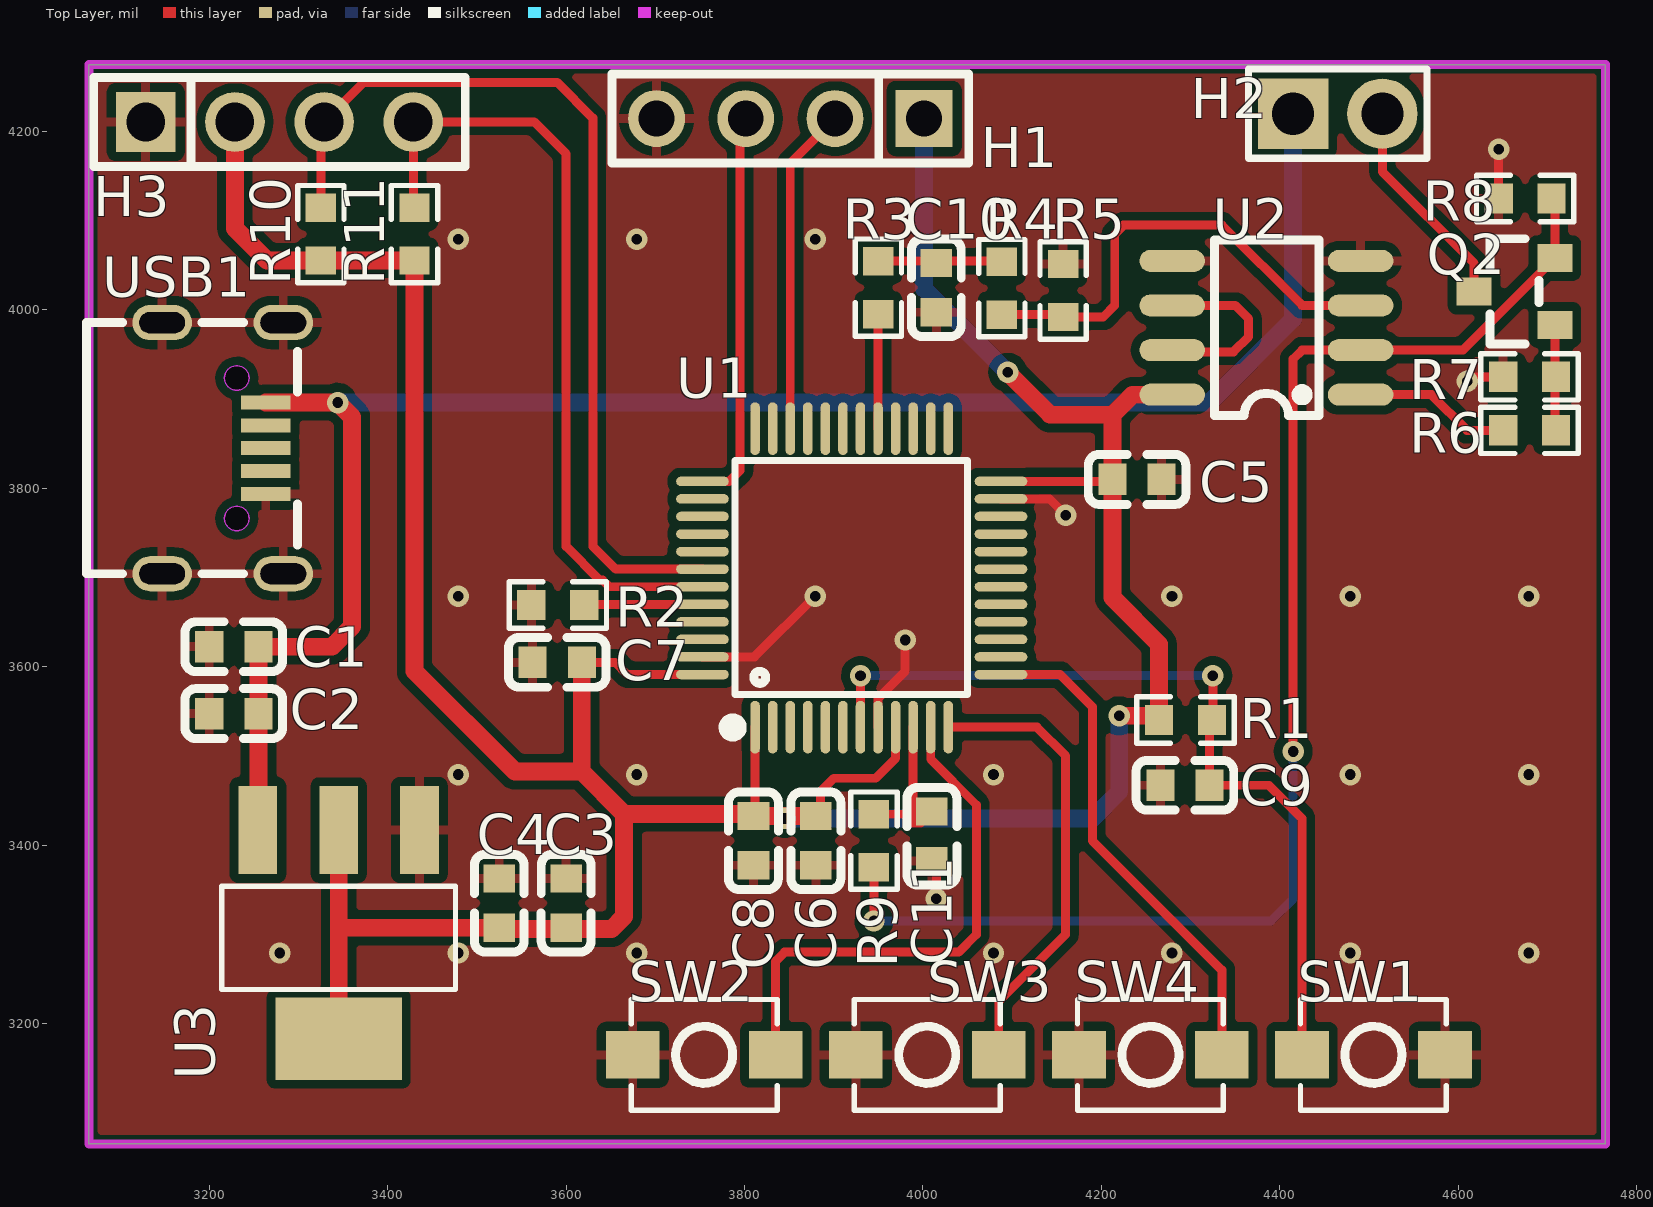
[diagram p0: Top Layer view]
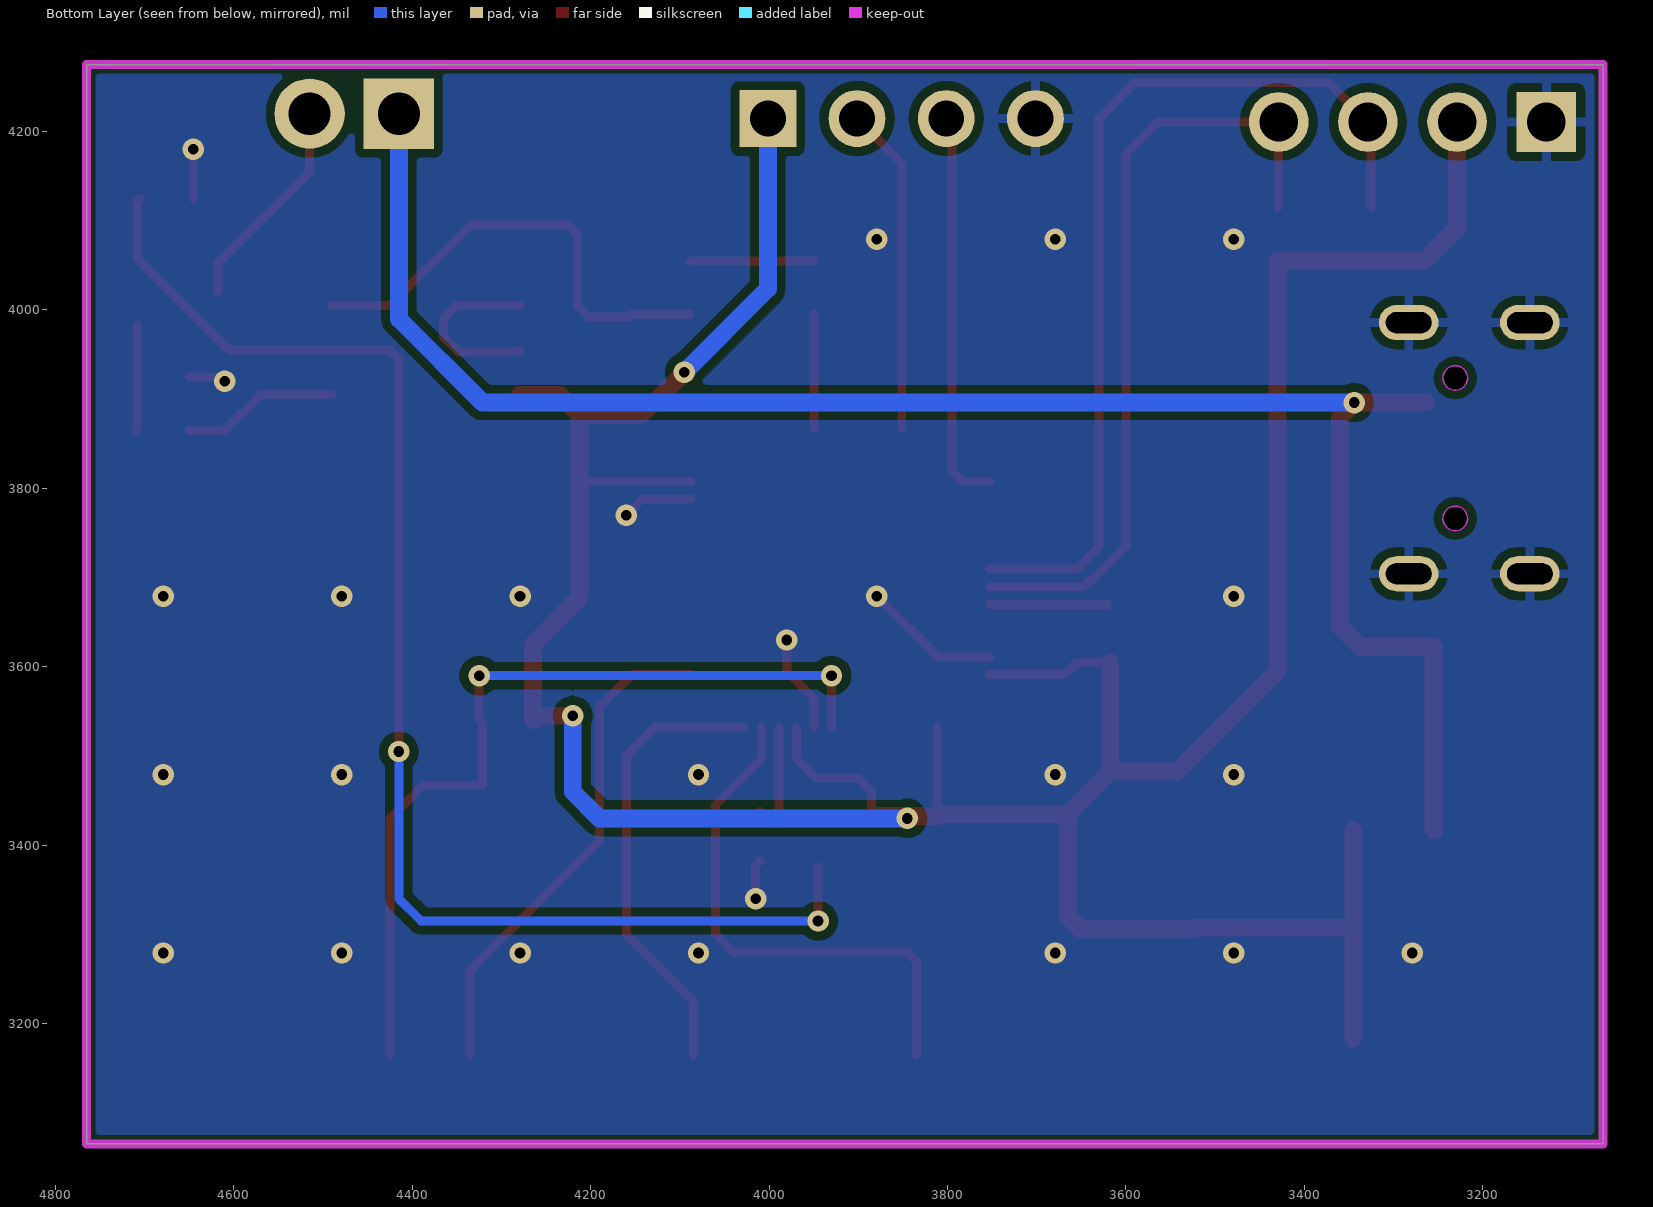
[diagram p1: Bottom Layer view, seen from below]
# Altium PCB MISC52008.pcbdoc
Units mil, origin at the board's own origin, x right, y up, seen from the top; angles counter-clockwise.
Board outline 1700 x 1210 mil, 2 copper layers (Top Layer, Bottom Layer), stack 62.206 mil thick; 34 components, 21 nets, 134 pads, 33 vias.

## Layer stack, top to bottom
Top Solder Mask Layer: solder mask 0.394, Dk 3.3
Top Layer: signal copper 1.379
Dielectric1: surface 59.449, FR4, Dk 4.5
Bottom Layer: signal copper 1.378
Bottom Solder Mask Layer: solder mask 0.394, Dk 3.3

## Board outline
3065,4275 3065,3065 4765,3065 4765,4275

## Design rules (kind name [scope] priority, off if disabled: settings)
BoardOutlineClearance copperThickness2oz_1 [All] p2 off: genericclearance=7.99 ignorepadtopadclearanceinfootprint=FALSE except(0: Arc-SplitContinuation Track-SplitContinuation SMDPad-SplitContinuation THPad-SplitContinuation Via-SplitContinuation Fill-SplitContinuation Region-SplitContinuation Poly-SplitContinuation Text-SplitContinuation Hole-SplitContinuation; 5.98: Arc-CutoutEdge SMDPad-CutoutEdge THPad-CutoutEdge Via-CutoutEdge Fill-CutoutEdge Region-CutoutEdge Text-CutoutEdge; 6.93: Hole-OutlineEdge Hole-CutoutEdge; 10: Poly-OutlineEdge Poly-CutoutEdge; 11.81: Arc-OutlineEdge Track-OutlineEdge SMDPad-OutlineEdge THPad-OutlineEdge Via-OutlineEdge Fill-OutlineEdge Region-OutlineEdge Text-OutlineEdge Track-CutoutEdge)
BoardOutlineClearance copperThickness1oz_1 [All] p4: genericclearance=4.02 ignorepadtopadclearanceinfootprint=FALSE except(0: Arc-SplitContinuation Track-SplitContinuation SMDPad-SplitContinuation THPad-SplitContinuation Via-SplitContinuation Fill-SplitContinuation Region-SplitContinuation Poly-SplitContinuation Text-SplitContinuation Hole-SplitContinuation; 6: SMDPad-CutoutEdge THPad-CutoutEdge Via-CutoutEdge Fill-CutoutEdge Region-CutoutEdge Text-CutoutEdge; 6.93: Hole-OutlineEdge Hole-CutoutEdge; 10: Poly-OutlineEdge Poly-CutoutEdge; 11.8: Arc-OutlineEdge Track-OutlineEdge SMDPad-OutlineEdge THPad-OutlineEdge Via-OutlineEdge Fill-OutlineEdge Region-OutlineEdge Text-OutlineEdge; 11.81: Arc-CutoutEdge Track-CutoutEdge)
Clearance copperThickness2oz [All] p1 off: gap=7.99 ignorepadtopadclearanceinfootprint=FALSE except(5.98: SMDPad-Track SMDPad-SMDPad THPad-Track SMDPad-THPad THPad-THPad Track-Via SMDPad-Via THPad-Via Via-Via Fill-Track Region-Track Fill-SMDPad Region-SMDPad Fill-THPad Region-THPad Fill-Via Region-Via Fill-Fill Fill-Region Region-Region Arc-Track Arc-SMDPad Arc-THPad Arc-Via Fill-Arc Region-Arc Arc-Arc Text-Track SMDPad-Text Text-THPad Text-Via Fill-Text Region-Text Arc-Text Text-Text; 6.93: Hole-Track Hole-SMDPad Hole-THPad Hole-Via Fill-Hole Region-Hole Hole-Arc Hole-Text; 10: Poly-Track Poly-SMDPad Poly-THPad Poly-Via Poly-Fill Poly-Region Poly-Poly Poly-Arc Poly-Text Poly-Hole)
Clearance copperThickness1oz [All] p3: gap=4.02 ignorepadtopadclearanceinfootprint=FALSE except(5.98: SMDPad-Track SMDPad-SMDPad THPad-Track SMDPad-THPad THPad-THPad Track-Via SMDPad-Via THPad-Via Via-Via Fill-Track Region-Track Fill-SMDPad Region-SMDPad Fill-THPad Region-THPad Fill-Via Region-Via Fill-Fill Fill-Region Region-Region; 6: Arc-Track Arc-SMDPad Arc-THPad Arc-Via Fill-Arc Region-Arc Arc-Arc Text-Track SMDPad-Text Text-THPad Text-Via Fill-Text Region-Text Arc-Text Text-Text; 6.93: Hole-Track Hole-SMDPad Hole-THPad Hole-Via Fill-Hole Region-Hole Hole-Arc Hole-Text; 10: Poly-Track Poly-SMDPad Poly-THPad Poly-Via Poly-Fill Poly-Region Poly-Poly Poly-Arc Poly-Text Poly-Hole)
DiffPairsRouting differentialPair [All] p1: maxlimit=6 minlimit=6 mostfreqgap=6 toplayer_minwidth=5 toplayer_prefwidth=10 toplayer_maxwidth=100 toplayer_mingap=6 toplayer_prefgap=6 toplayer_maxgap=6 bottomlayer_minwidth=5 bottomlayer_prefwidth=10 bottomlayer_maxwidth=100 bottomlayer_mingap=6 bottomlayer_prefgap=6 bottomlayer_maxgap=6 maxuncoupledlength=10
HoleToHoleClearance otherClearance [All] p1: gap=11.81 allowstackedmicrovias=TRUE
Length netLength [All] p1: minlimit=0 maxlimit=0
MatchedLengths netLengthTolerance [All] p1: tolerance=1000
PasteMaskExpansion pasteMaskExpansion [All] p1: expansion=0
PlaneConnect innerPlane [All] p1: planeconnectstyle=Relief reliefexpansion=20 reliefentries=4 reliefconductorwidth=10 reliefairgap=10
PolygonConnect copperRegion [(InNet('GND'))] p1: connectstyle=Relief reliefconductorwidth=10 reliefentries=4 polygonreliefangle="90 Angle" airgapwidth=10 via.connectstyle=Relief via.reliefconductorwidth=10 via.reliefentries=4 via.polygonreliefangle="90 Angle" via.airgapwidth=10
RoutingVias viaSize [All] p1: holewidth=12.01 width=24.02 viastyle="Through Hole" minholewidth=11.81 minwidth=19.68 maxholewidth=248.03 maxwidth=393.7
SolderMaskExpansion solderMaskExpansion [IsVia] p1: expansion=-1000 istentingtop=TRUE
SolderMaskExpansion solderMaskExpansion [All] p2: expansion=2 istentingtop=FALSE
Width copperThickness2oz_2 [All] p1 off: maxlimit=100 minlimit=8 preferedwidth=10
Width copperThickness1oz_2 [All] p2: maxlimit=100 minlimit=5 preferedwidth=10

## Components (designator, comment, footprint, x,y, rotation, side; value= is the part's Value field where it differs from the comment)
C1 "10uf" C0603 3227.5,3622.5 r0 top
C2 "0.1uf" C0603 3227.5,3547.5 r0 top
C3 "10uf" C0603 3600,3335 r270 top
C4 "0.1uf" C0603 3525,3335 r270 top
C5 "0.1uf" C0603 4240,3810 r180 top
C6 "0.1uf" C0603 3880,3405 r90 top
C7 "0.1uf" C0603 3590,3605 r0 top
C8 "0.1uf" C0603 3810,3405 r90 top
C9 "0.1uf" C0603 4293.67,3467.16 r0 top
C10 "1uf" C0603 4015,4025 r270 top
C11 "100nF" C0603 4010,3410 r90 top
H1 "HX PH254-01-04-Z-L11.5 straight pin header" HDR-TH_4P-HX-PH254-01-04-Z-L11.5 3851.34,4214.55 r180 top
H2 "HX PH254-01-02-Z-L11.5 male header connector" HDR-TH_2P-P2.54-V-M 4465,4220 r0 top
H3 "2.54-1*4P female" HDR-TH_4P-P2.54-V-F 3278.67,4210.72 r0 top
Q2 "AO3400" SOT-23_L2.9-W1.3-P1.90-LS2.4-BR 4663.04,4020.72 r0 top
R1 "10K" R0603 4294.35,3540.26 r180 top
R2 "100K" R0603 3590.66,3669.2 r180 top
R3 "10K" R0603 3950,4025 r90 top
R4 "3.3k" R0603 4088.39,4024.39 r270 top
R5 "5.1k" R0603 4157.2,4021.75 r90 top
R6 "100" R0603 4680,3865 r0 top
R7 "100K" R0603 4680,3925 r0 top
R8 "10K" R0603 4675,4125 r0 top
R9 "10K" R0603 3945,3405 r90 top
R10 "4.7K" R0603 3325,4085 r90 top
R11 "4.7K" R0603 3430,4085 r90 top
SW1 "" Key_SMD_3x4x2 4505,3165 r0 top
SW2 "" Key_SMD_3x4x2 3754.79,3165 r180 top
SW3 "" Key_SMD_3x4x2 4004.86,3165 r180 top
SW4 "" Key_SMD_3x4x2 4254.93,3165 r180 top
U1 "AT32F421C8T7" LQFP-48_L7.0-W7.0-P0.50-LS9.0-BL 3920.11,3699.55 r0 top
U2 "LMV358" SOP-8_L4.9-W3.9-P1.27-LS6.0-BL 4385,3980 r90 top
U3 "AMS1117-3.3(XBLW)" SOT-223-3_L6.5-W3.4-P2.30-LS7.0-BR-1 3345,3300 r90 top
USB1 "" USB_Micro 3215,3845 r270 top

## Footprints (in the part's own frame and the unit in brackets; to place one, negate y for a bottom-side part, rotate by r counter-clockwise, add the part's x,y. Pads: shape width x height; smd on the part's side, far side on the other; paste and mask are expansions set on the pad)
C0603 [mm]
  rect 0.8x0.9 smd: 1(-0.7,0) 2(0.7,0)
  silkscreen extent -1.39,-0.71 1.39,0.71
HDR-TH_2P-P2.54-V-M [mm]
  rect 2x2 hole 1.2: 1(-1.27,0)
  round 2 hole 1.2: 2(1.27,0)
  silkscreen extent -2.54,-1.27 2.54,1.27
HDR-TH_4P-HX-PH254-01-04-Z-L11.5 [mm]
  rect 1.62x1.62 hole 1.02: 1(-3.81,0)
  round 1.62 hole 1.02: 2(-1.27,0) 3(1.27,0) 4(3.81,0)
  silkscreen extent -5.08,-1.27 5.08,1.27
HDR-TH_4P-P2.54-V-F [mm]
  rect 1.7x1.7 hole 1.1: 1(-3.81,0)
  round 1.7 hole 1.1: 2(-1.27,0) 3(1.27,0) 4(3.81,0)
  silkscreen extent -5.29,-1.27 5.29,1.27
Key_SMD_3x4x2 [mm]
  rect 1.53x1.36 smd paste+0 mask+0.051: 1(-2.035,0) 2(2.035,0)
  silkscreen extent -2.08,-1.58 2.08,1.58
LQFP-48_L7.0-W7.0-P0.50-LS9.0-BL [mm]
  oval 0.27x1.5 smd paste+0 mask+0.05: 1(-2.75,-4.25) 2(-2.25,-4.25) 3(-1.75,-4.25) 4(-1.25,-4.25) 5(-0.75,-4.25) 6(-0.25,-4.25) 7(0.25,-4.25) 8(0.75,-4.25) 9(1.25,-4.25) 10(1.75,-4.25) 11(2.25,-4.25) 12(2.75,-4.25) 25(2.75,4.25) 26(2.25,4.25) 27(1.75,4.25) 28(1.25,4.25) 29(0.75,4.25) 30(0.25,4.25) 31(-0.25,4.25) 32(-0.75,4.25) 33(-1.25,4.25) 34(-1.75,4.25) 35(-2.25,4.25) 36(-2.75,4.25)
  oval 1.5x0.27 smd paste+0 mask+0.05: 13(4.25,-2.75) 14(4.25,-2.25) 15(4.25,-1.75) 16(4.25,-1.25) 17(4.25,-0.75) 18(4.25,-0.25) 19(4.25,0.25) 20(4.25,0.75) 21(4.25,1.25) 22(4.25,1.75) 23(4.25,2.25) 24(4.25,2.75) 37(-4.25,2.75) 38(-4.25,2.25) 39(-4.25,1.75) 40(-4.25,1.25) 41(-4.25,0.75) 42(-4.25,0.25) 43(-4.25,-0.25) 44(-4.25,-0.75) 45(-4.25,-1.25) 46(-4.25,-1.75) 47(-4.25,-2.25) 48(-4.25,-2.75)
  silkscreen extent -3.59,-4.46 3.3,3.34
R0603 [mil]
  rect 31.75x34.02 smd paste-3937.01 mask+2: 1(-29.66,0) 2(29.66,0)
  silkscreen extent -55,-26 55,26
SOP-8_L4.9-W3.9-P1.27-LS6.0-BL [mm]
  oval 0.63x1.865 smd: 1(-1.905,-2.682) 2(-0.635,-2.682) 3(0.635,-2.682) 4(1.905,-2.682) 5(1.905,2.682) 6(0.635,2.682) 7(-0.635,2.682) 8(-1.905,2.682)
  silkscreen extent -2.5,-1.5 2.5,1.48
SOT-23_L2.9-W1.3-P1.90-LS2.4-BR [mm]
  rect 1x0.8 smd: 1(1.15,-0.95) 2(1.15,0.95) 3(-1.15,0)
  silkscreen extent -0.7,-1.5 0.7,1.5
SOT-223-3_L6.5-W3.4-P2.30-LS7.0-BR-1 [mm]
  rect 2.5x1.1 smd: 1(2.97,-2.3) 2(2.97,0) 3(2.97,2.3)
  rect 2.34x3.6 smd: 2(-2.97,0)
  silkscreen extent -1.57,-3.33 1.37,3.33
USB_Micro [mm]
  rect 0.4x1.4 smd paste-100 mask+0.05: 1(-1.3,1.225) 2(-0.65,1.225) 3(0,1.225) 4(0.65,1.225) 5(1.3,1.225)
  oval 1x1.7 hole 0.6 slot 1.3 at 90 deg paste+0 mask+0.05: 6(-3.575,-1.725) 6(-3.575,1.725) 6(3.575,-1.725) 6(3.575,1.725)
  Board Outline Layer circle w0.003: c-2,0.4 r0.35
  Board Outline Layer circle w0.003: c2,0.4 r0.35
  Board Outline Layer region: -2,0.75 -1.848,0.715 -1.726,0.618 -1.659,0.478 -1.659,0.322 -1.726,0.182 -1.848,0.085 -2,0.05 -2,0.05 -2.152,0.085 -2.274,0.182 -2.341,0.322 -2.341,0.478 -2.274,0.618 -2.152,0.715 -2,0.75
  Board Outline Layer region: -2,0.75 -1.922,0.741 -1.848,0.715 -1.782,0.674 -1.726,0.618 -1.685,0.552 -1.659,0.478 -1.65,0.4 -1.659,0.322 -1.685,0.248 -1.726,0.182 -1.782,0.126 -1.848,0.085 -1.922,0.059 -2,0.05 -2.078,0.059 -2.152,0.085 -2.218,0.126 -2.274,0.182 -2.315,0.248 -2.341,0.322 -2.35,0.4 -2.341,0.478 -2.315,0.552 -2.274,0.618 -2.218,0.674 -2.152,0.715 -2.078,0.741
  Board Outline Layer region: 2,0.75 2.152,0.715 2.274,0.618 2.341,0.478 2.341,0.322 2.274,0.182 2.152,0.085 2,0.05 2,0.05 1.848,0.085 1.726,0.182 1.659,0.322 1.659,0.478 1.726,0.618 1.848,0.715 2,0.75
  Board Outline Layer region: 2,0.75 2.078,0.741 2.152,0.715 2.218,0.674 2.274,0.618 2.315,0.552 2.341,0.478 2.35,0.4 2.341,0.322 2.315,0.248 2.274,0.182 2.218,0.126 2.152,0.085 2.078,0.059 2,0.05 1.922,0.059 1.848,0.085 1.782,0.126 1.726,0.182 1.685,0.248 1.659,0.322 1.65,0.4 1.659,0.478 1.685,0.552 1.726,0.618 1.782,0.674 1.848,0.715 1.922,0.741
  Multi-Layer board cut-out: -2,0.75 -1.848,0.715 -1.726,0.618 -1.659,0.478 -1.659,0.322 -1.726,0.182 -1.848,0.085 -2,0.05 -2,0.05 -2.152,0.085 -2.274,0.182 -2.341,0.322 -2.341,0.478 -2.274,0.618 -2.152,0.715 -2,0.75
  Multi-Layer board cut-out: 2,0.75 2.152,0.715 2.274,0.618 2.341,0.478 2.341,0.322 2.274,0.182 2.152,0.085 2,0.05 2,0.05 1.848,0.085 1.726,0.182 1.659,0.322 1.659,0.478 1.726,0.618 1.848,0.715 2,0.75
  silkscreen extent -3.57,-3.87 3.57,2.14

## Via types
v1: diameter 24.02, hole 12, Top Layer to Bottom Layer, 33 vias

## Nets (pads, with @x,y where several pads share a name; then routed paths per layer and width w, separated by ;. In a path a pad name is that pad's centre, name@x,y a point inside that pad or via, vN(x,y) a via of type N, cw(c..) or ccw(c..) an arc to the next point about the centre after c; other vN are vias at no path point)
$1N142: R3.1 U1.29 | length 128.6
  Top Layer w10: U1.29 3949.64,3994.98 R3.1
$1N161: U2.6 U2.7 | length 205.4
  Top Layer w10: U2.7 4281.46,3952.93 4347.93,3952.93 4365,3970 4365,3990 4350,4005 U2.6
$1N163: Q2.1 R6.2 R7.2 | length 118.9
  Top Layer w10: Q2.1 4708.31,3866.35 R6.2
+3V3: C3.2 C4.2 C5.2 C6.2 C7.2 C8.2 H1.1 H3.2 R1.2 R10.1 R11.1 U1.1 U1.9 U1.24 U1.48 U2.8 U3.2 | length 4062.3
  Top Layer w10: C7.2 3655,3605 3668.72,3591.28 U1.48 ; C8.2 3811.84,3434.4 U1.1 ; C6.2 3885,3437.56 3885,3460 3900,3475 3946.92,3475 3969.32,3497.4 U1.9 ; U1.24 4202.82,3807.82 4205,3810 C5.2
  Top Layer w20: H3.2 3228.67,4091.33 3264.66,4055.34 R10.1 R11.1 3430,3595 3542.56,3482.44 3617.56,3482.44 ; U3.2@3345,3183.07 3345,3307.44 ; U3.2@3345,3416.93 3345,3307.44 ; C7.2 3617.56,3482.44 ; C6.2 C8.2 3807.56,3435 3665,3435 ; v1(4095,3930) 4142.56,3882.44 4212.44,3882.44 ; v1(4220,3545) 4259.95,3545 R1.2 4264.69,3625.31 4212.44,3677.56 C5.2 4212.44,3882.44 ; U2.8 4235,3905 4212.44,3882.44 ; 3345,3307.44 C4.2 3526.58,3305.86 3650.86,3305.86 3665,3320 3665,3435 ; 3617.56,3482.44 3665,3435
  Bottom Layer w20: v1(3845,3430) 4190,3430 4220,3460 v1(4220,3545) ; H1.1 4001.34,4023.66 v1(4095,3930)
+5V: C1.2 C2.2 H2.1 U3.3 USB1.1 | length 1998.6
  Top Layer w20: U3.3 3255.06,3417.53 C2.2 C1.2 3337.5,3622.5 3360,3645 3360,3880 v1(3343.82,3896.18) USB1.1
  Bottom Layer w20: v1(3343.82,3896.18) 4321.18,3896.18 4415,3990 H2.1
BOOT0: R2.1 U1.44 | length 132.8
  Top Layer w10: R2.1 3621.14,3670.02 U1.44
GND: C1.1 C2.1 C3.1 C4.1 C5.1 C6.1 C7.1 C8.1 C9.1 C10.2 C11.1 H1.4 H3.1 R2.2 R5.2 R7.1 R8.1 SW1.2 SW2.2 SW3.2 SW4.2 U1.8 U1.23 U1.47 U2.4 U2.5 U3.1 USB1.5 USB1.6 | length 486.9
  Top Layer w10: U1.47 3810.97,3610.97 v1(3879.1,3679.1) ; U1.8 3949.64,3564.64 3980,3595 v1(3980,3630) ; C11.1 4015,3377.44 v1(4015,3340) ; U1.23 4141.87,3788.13 v1(4160,3770) ; v1(4610,3920) 4615,3925 R7.1 ; R8.1 v1(4645.34,4180)
  other v1: 3279.1,3279.1 3479.1,3279.1 3679.1,3279.1 4079.1,3279.1 4279.1,3279.1 4479.1,3279.1 4679.1,3279.1 3479.1,3479.1 3679.1,3479.1 4079.1,3479.1 4479.1,3479.1 4679.1,3479.1 3479.1,3679.1 4279.1,3679.1 4479.1,3679.1 4679.1,3679.1 3479.1,4079.1 3679.1,4079.1 3879.1,4079.1
NRES: C9.2 R1.1 SW1.1 U1.7 | length 961.3
  Top Layer w10: U1.7 v1(3929.95,3590) ; v1(4325,3590) 4325,3541.25 R1.1 4321.23,3537.48 C9.2 4387.84,3467.16 4424.88,3430.12 SW1.1
  Bottom Layer w10: v1(3929.95,3590) v1(4325,3590)
OUT-: H2.2 Q2.3 | length 241.8
  Top Layer w10: H2.2 4515,4155 4617.76,4052.24 Q2.3
OUTA: R6.1 U2.1 | length 176.3
  Top Layer w10: U2.1 4570,3905 4610,3865 R6.1
PA0: C11.2 R9.2 U1.10 | length 182.1
  Top Layer w10: R9.2 3979.01,3434.66 3989.01,3424.66 ; U1.10 3989.01,3424.66 ; C11.2 3997.1,3424.66 3989.01,3424.66
PA1: SW2.1 U1.11 | length 596
  Top Layer w10: SW2.1 3834.91,3270 3844.91,3280 4040,3280 4060,3300 4060,3445 4008.69,3496.31 U1.11
PA2: SW3.1 U1.12 | length 511
  Top Layer w10: U1.12 4127.77,3532.23 4160,3500 4160,3300 4084.98,3224.98 SW3.1
PA3: SW4.1 U1.13 | length 567.7
  Top Layer w10: U1.13 4153.72,3591.28 4190,3555 4190,3405 4335.05,3259.95 SW4.1
PWM_F: C10.1 R3.2 R4.1 | length 138.6
  Top Layer w10: R3.2 4087.78,4054.66 R4.1
SCL: H3.3 R10.2 U1.42 | length 1047.4
  Top Layer w10: R10.2 3325,4207.05 H3.3 3373.12,4255.17 3589.83,4255.17 3630,4215 3630,3735 3655.61,3709.39 U1.42
SDA: H3.4 R11.2 U1.43 | length 894.3
  Top Layer w10: R11.2 3428.67,4115.99 H3.4 3564.28,4210.72 3600,4175 3600,3735 3637.81,3697.19 3640.75,3697.19 3648.23,3689.71 U1.43
SWCLK: H1.3 U1.37 | length 444.4
  Top Layer w10: U1.37 3782.82,3807.82 3795,3820 3795,4208.21 H1.3
SWDIO: H1.2 U1.34 | length 368.4
  Top Layer w10: U1.34 3851.21,4164.42 H1.2
VREF: R4.2 R5.1 U2.3 | length 530.1
  Top Layer w10: R4.2 4154.56,3994.73 R5.1 4202.09,3992.09 4215,4005 4215,4085 4225,4095 4335,4095 4425,4005 U2.3
VSENSE: Q2.2 R8.2 R9.1 U2.2 | length 1554.3
  Top Layer w10: v1(3945,3315) R9.1 ; v1(4415,3505) 4415,3945 4425,3955 U2.2 4605.19,3955 Q2.2 4708.31,4121.35 R8.2
  Bottom Layer w10: v1(3945,3315) 4390,3315 4415,3340 v1(4415,3505)
pads on no net: U1.2 U1.3 U1.4 U1.5 U1.6 U1.14 U1.15 U1.16 U1.17 U1.18 U1.19 U1.20 U1.21 U1.22 U1.25 U1.26 U1.27 U1.28 U1.30 U1.31 U1.32 U1.33 U1.35 U1.36 U1.38 U1.39 U1.40 U1.41 U1.45 U1.46 USB1.2 USB1.3 USB1.4

## Polygon pours and split planes (outlines as drawn)
GND on Top Layer (solid, remove dead copper, pour order 0): 3020,4355 3020,3015 4860,3015 4860,4355
GND on Bottom Layer (solid, remove dead copper, pour order 2): 3000,4335 3000,3000 4865,3000 4865,4335

## Keep-outs
Board Outline Layer:
  the board outline again, w10